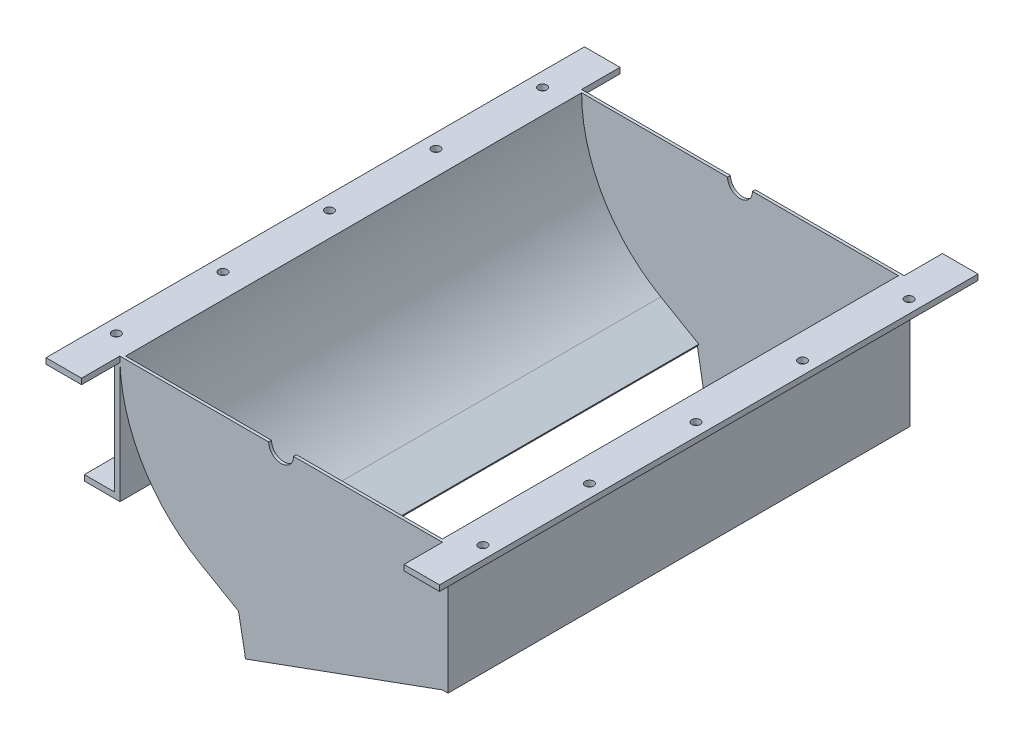
from build123d import *

# Parameters (mm, degrees)
BOSS_EXTRUDE2_DEPTH       = 325
BOSS_EXTRUDE2_2_DEPTH     = 325
BOSS_EXTRUDE3_DEPTH       = 4
BOSS_EXTRUDE4_START       = -4
BOSS_EXTRUDE4_DEPTH       = 4
SKETCH5_R                 = 6
CUT_EXTRUDE1_DEPTH        = 10
LPATTERN1_COUNT           = 3
LPATTERN1_PITCH           = 150
LPATTERN2_COPY_1_SKETCH_R = 6
LPATTERN2_COPY_1_DEPTH    = 10
LPATTERN2_COPY_2_SKETCH_R = 6
LPATTERN2_COPY_2_DEPTH    = 10
LPATTERN2_COPY_3_SKETCH_R = 6
LPATTERN2_COPY_3_DEPTH    = 10
LPATTERN2_COPY_4_SKETCH_R = 6
LPATTERN2_COPY_4_DEPTH    = 10
LPATTERN2_COPY_5_SKETCH_R = 6
LPATTERN2_COPY_5_DEPTH    = 10
LPATTERN2_COPY_6_SKETCH_R = 6
LPATTERN2_COPY_6_DEPTH    = 10
CUT_EXTRUDE2_DEPTH        = 762.052386329
CUT_EXTRUDE2_DEPTH_BACK   = 762.052386329
SKETCH6_R                 = 17.5
CUT_EXTRUDE3_DEPTH        = 762.052386329
CUT_EXTRUDE3_DEPTH_BACK   = 762.052386329
SKETCH7_W                 = 100.370226039
SKETCH7_H                 = 50
SKETCH8_W                 = 650
SKETCH8_H                 = 8
BOSS_EXTRUDE5_DEPTH       = 42.141012962
CUT_EXTRUDE4_DEPTH        = 762.052386329
CUT_EXTRUDE4_DEPTH_BACK   = 762.052386329
SKETCH9_W                 = 99.024260435
SKETCH9_H                 = 85.798945111
SKETCH10_W                = 50
SKETCH10_H                = 54
BOSS_EXTRUDE6_DEPTH       = 8


with BuildPart() as part:
    # Sketch1 → Boss-Extrude2 (new, symmetric)
    with BuildSketch(Plane.XY):
        with BuildLine():
            Line((-223, 0), (-277, 0))
            Line((-277, 0), (-277, -8))
            Line((-277, -8), (-234.858987038, -8))
            Line((-234.858987038, -8), (-234.858987038, -219.476006061))
            Line((-234.858987038, -219.476006061), (-278.858987038, -219.476006061))
            Line((-278.858987038, -219.476006061), (-278.858987038, -227.476006061))
            Line((-278.858987038, -227.476006061), (-226.858987038, -227.476006061))
            Line((-226.858987038, -227.476006061), (-226.858987038, -8))
            ThreePointArc((-226.858987038, -8), (-194.556923413, -116.947011728), (-113.5, -196.587766659))
            Line((-113.5, -196.587766659), (-60, -227.476006061))
            Line((-60, -227.476006061), (-58, -224.011904446))
            Line((-58, -224.011904446), (-111.5, -193.123665044))
            ThreePointArc((-111.5, -193.123665044), (-193.123665044, -111.5), (-223, 0))
        make_face()
    extrude(amount=BOSS_EXTRUDE2_DEPTH, both=True)



with BuildPart() as body_2:
    # Sketch1 → Boss-Extrude2 2 (new, symmetric)
    with BuildSketch(Plane.XY):
        Polygon((277, 0), (223, 0), (223, -177.199169847), (-51.368080573, -277.060984409), (-50, -280.819754892), (227, -180), (227, -227.476006061), (279, -227.476006061), (279, -219.476006061), (235, -219.476006061), (235, -8), (277, -8), align=None)
    extrude(amount=BOSS_EXTRUDE2_2_DEPTH, both=True)


with BuildPart() as part_1:
    add(part.part)

    add(body_2.part)  # Boss-Extrude3 merges body 2
    # Sketch3 → Boss-Extrude3 (add)
    with BuildSketch(Plane.XY.offset(325)):
        with BuildLine():
            Line((-58, -224.011904446), (-60, -227.476006061))
            Line((-60, -227.476006061), (84.865527782, -227.476006061))
            Line((84.865527782, -227.476006061), (223, -177.199169847))
            Line((223, -177.199169847), (223, 0))
            Line((223, 0), (-223, 0))
            ThreePointArc((-223, 0), (-193.123665044, -111.5), (-111.5, -193.123665044))
            Line((-111.5, -193.123665044), (-58, -224.011904446))
        make_face()
        Polygon((84.865527782, -227.476006061), (-60, -227.476006061), (-50.747008298, -276.834932587), align=None)
    extrude(amount=-BOSS_EXTRUDE3_DEPTH)

    # Sketch4 → Boss-Extrude4 (add)
    with BuildSketch(Plane(origin=(0, 0, -325), x_dir=(-1, 0, 0), z_dir=(0, 0, -1)).offset(BOSS_EXTRUDE4_START)):
        with BuildLine():
            Line((111.5, -193.123665044), (58, -224.011904446))
            Line((58, -224.011904446), (60, -227.476006061))
            Line((60, -227.476006061), (51.368080573, -277.060984409))
            Line((51.368080573, -277.060984409), (-223, -177.199169847))
            Line((-223, -177.199169847), (-223, 0))
            Line((-223, 0), (223, 0))
            ThreePointArc((223, 0), (193.123665044, -111.5), (111.5, -193.123665044))
        make_face()
    extrude(amount=BOSS_EXTRUDE4_DEPTH)

    # Sketch5 → Cut-Extrude1 (cut)
    with BuildSketch(Plane(origin=(0, 0, 0), x_dir=(1, 0, 0), z_dir=(0, 1, 0))):
        with Locations(Location((-257, 0, 0), (0, 0, 180))):
            Circle(SKETCH5_R)
        with Locations(Location((259, 0, 0), (0, 0, 180))):
            Circle(SKETCH5_R)
    cut_extrude1 = extrude(amount=-CUT_EXTRUDE1_DEPTH, mode=Mode.SUBTRACT)

    # LPattern1: Cut-Extrude1 ×3
    with Locations(*[(0, 0, -i * LPATTERN1_PITCH) for i in range(1, LPATTERN1_COUNT)]):
        add(cut_extrude1, mode=Mode.SUBTRACT)

    # LPattern2 copy 1 sketch → LPattern2 copy 1 (cut)
    with BuildSketch(Plane(origin=(0, 0, 0), x_dir=(1, 0, 0), z_dir=(0, 1, 0))):
        with Locations(Location((-257, 0, 0), (0, 0, 180))):
            Circle(LPATTERN2_COPY_1_SKETCH_R)
        with Locations(Location((259, 0, 0), (0, 0, 180))):
            Circle(LPATTERN2_COPY_1_SKETCH_R)
    extrude(amount=-LPATTERN2_COPY_1_DEPTH, mode=Mode.SUBTRACT)

    # LPattern2 copy 2 sketch → LPattern2 copy 2 (cut)
    with BuildSketch(Plane(origin=(0, 0, 150), x_dir=(1, 0, 0), z_dir=(0, 1, 0))):
        with Locations(Location((-257, 0, 0), (0, 0, 180))):
            Circle(LPATTERN2_COPY_2_SKETCH_R)
        with Locations(Location((259, 0, 0), (0, 0, 180))):
            Circle(LPATTERN2_COPY_2_SKETCH_R)
    extrude(amount=-LPATTERN2_COPY_2_DEPTH, mode=Mode.SUBTRACT)

    # LPattern2 copy 3 sketch → LPattern2 copy 3 (cut)
    with BuildSketch(Plane(origin=(0, 0, -150), x_dir=(1, 0, 0), z_dir=(0, 1, 0))):
        with Locations(Location((-257, 0, 0), (0, 0, 180))):
            Circle(LPATTERN2_COPY_3_SKETCH_R)
        with Locations(Location((259, 0, 0), (0, 0, 180))):
            Circle(LPATTERN2_COPY_3_SKETCH_R)
    extrude(amount=-LPATTERN2_COPY_3_DEPTH, mode=Mode.SUBTRACT)

    # LPattern2 copy 4 sketch → LPattern2 copy 4 (cut)
    with BuildSketch(Plane(origin=(0, 0, 0), x_dir=(1, 0, 0), z_dir=(0, 1, 0))):
        with Locations(Location((-257, 0, 0), (0, 0, 180))):
            Circle(LPATTERN2_COPY_4_SKETCH_R)
        with Locations(Location((259, 0, 0), (0, 0, 180))):
            Circle(LPATTERN2_COPY_4_SKETCH_R)
    extrude(amount=-LPATTERN2_COPY_4_DEPTH, mode=Mode.SUBTRACT)

    # LPattern2 copy 5 sketch → LPattern2 copy 5 (cut)
    with BuildSketch(Plane(origin=(0, 0, 150), x_dir=(1, 0, 0), z_dir=(0, 1, 0))):
        with Locations(Location((-257, 0, 0), (0, 0, 180))):
            Circle(LPATTERN2_COPY_5_SKETCH_R)
        with Locations(Location((259, 0, 0), (0, 0, 180))):
            Circle(LPATTERN2_COPY_5_SKETCH_R)
    extrude(amount=-LPATTERN2_COPY_5_DEPTH, mode=Mode.SUBTRACT)

    # LPattern2 copy 6 sketch → LPattern2 copy 6 (cut)
    with BuildSketch(Plane(origin=(0, 0, 300), x_dir=(1, 0, 0), z_dir=(0, 1, 0))):
        with Locations(Location((-257, 0, 0), (0, 0, 180))):
            Circle(LPATTERN2_COPY_6_SKETCH_R)
        with Locations(Location((259, 0, 0), (0, 0, 180))):
            Circle(LPATTERN2_COPY_6_SKETCH_R)
    extrude(amount=-LPATTERN2_COPY_6_DEPTH, mode=Mode.SUBTRACT)

    # Sketch6 → Cut-Extrude2 (cut, two sides: drawn at the far end of the back side and taken through both)
    with BuildSketch(Plane(origin=(0, 0, -325), x_dir=(-1, 0, 0), z_dir=(0, 0, -1)).offset(-CUT_EXTRUDE2_DEPTH_BACK)):
        Circle(SKETCH6_R)
    extrude(amount=CUT_EXTRUDE2_DEPTH + CUT_EXTRUDE2_DEPTH_BACK, mode=Mode.SUBTRACT)

    # Sketch7 → Cut-Extrude3 (cut, two sides: drawn at the far end of the back side and taken through both)
    with BuildSketch(Plane.XY.offset(325).offset(-CUT_EXTRUDE3_DEPTH_BACK)):
        with Locations((-277.044100058, -202.476006061)):
            Rectangle(SKETCH7_W, SKETCH7_H)
    extrude(amount=CUT_EXTRUDE3_DEPTH + CUT_EXTRUDE3_DEPTH_BACK, mode=Mode.SUBTRACT)

    # Sketch8 → Boss-Extrude5 (add)
    with BuildSketch(Plane.ZY.offset(234.858987038)):
        with Locations((0, -173.476006061)):
            Rectangle(SKETCH8_W, SKETCH8_H)
    extrude(amount=BOSS_EXTRUDE5_DEPTH)

    # Sketch9 → Cut-Extrude4 (cut, two sides: drawn at the far end of the back side and taken through both)
    with BuildSketch(Plane.XY.offset(325).offset(-CUT_EXTRUDE4_DEPTH_BACK)):
        with Locations((276.512130218, -222.899472556)):
            Rectangle(SKETCH9_W, SKETCH9_H)
    extrude(amount=CUT_EXTRUDE4_DEPTH + CUT_EXTRUDE4_DEPTH_BACK, mode=Mode.SUBTRACT)

    # Sketch10 → Boss-Extrude6 (add)
    with BuildSketch(Plane(origin=(0, 0, 0), x_dir=(1, 0, 0), z_dir=(0, 1, 0))):
        with Locations((-252, 352)):
            Rectangle(SKETCH10_W, SKETCH10_H)
        with Locations((252, 352)):
            Rectangle(SKETCH10_W, SKETCH10_H)
        with Locations((252, -352)):
            Rectangle(SKETCH10_W, SKETCH10_H)
        with Locations((-252, -352)):
            Rectangle(SKETCH10_W, SKETCH10_H)
    extrude(amount=-BOSS_EXTRUDE6_DEPTH)


solid = part_1.part
